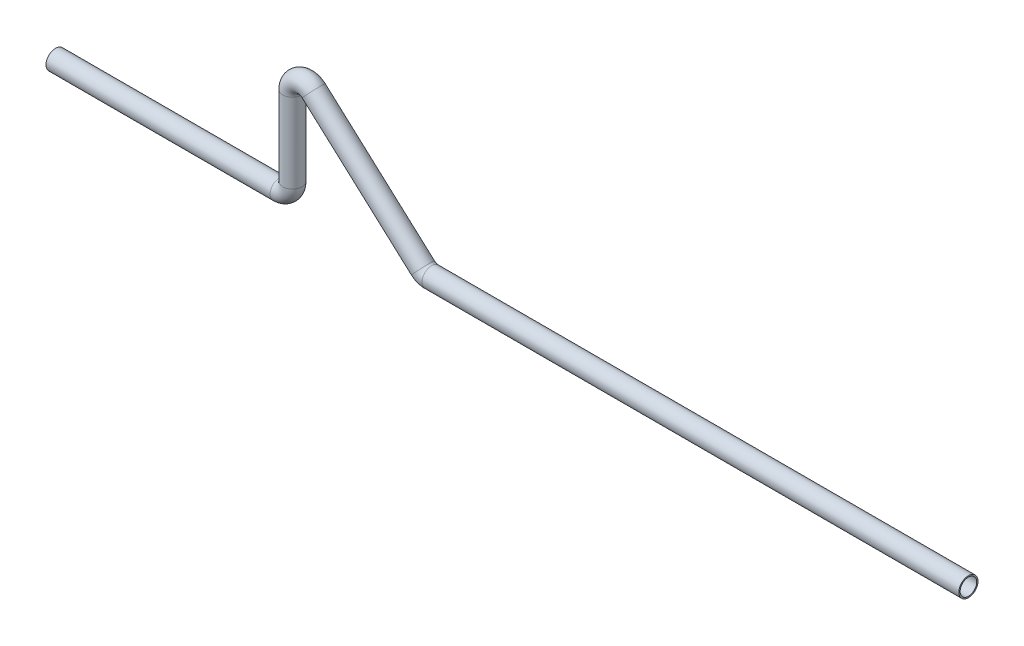
from build123d import *

# Parameters (mm, degrees)
SWEEP_THIN1_PROFILE_R   = 15
SWEEP_THIN1_PROFILE_R_2 = 13


with BuildPart() as part:
    # Sweep-Thin1: sweep along a curve in space
    with BuildLine() as sweep_thin1_path:
        Line((-2125, 3135.002861913, 100.000000001), (-1773.960788665, 3135.002861913, 100.000000001))
        ThreePointArc((-1773.960788665, 3135.002861913, 100.000000001), (-1759.818653041, 3140.860726289, 100.000000001), (-1753.960788665, 3155.002861913, 100.000000001))
        Line((-1753.960788665, 3155.002861913, 100.000000001), (-1753.960788665, 3279.60825422, 100.000000001))
        ThreePointArc((-1753.960788665, 3279.60825422, 100.000000001), (-1742.076616051, 3297.887568918, 100), (-1720.547454081, 3294.443430502, 100))
        Line((-1720.547454081, 3294.443430502, 100), (-1549.428219579, 3139.724706402, 99.999999999))
        ThreePointArc((-1536.014884995, 3134.559882685, 99.999999999), (-1543.201555794, 3135.895698727, 99.999999999), (-1549.428219579, 3139.724706402, 99.999999999))
        Line((-1536.014884995, 3134.559882685, 99.999999999), (-694.909600267, 3134.559882685, 99.999999999))
    # Sweep-Thin1 profile (on start of the path) → Sweep-Thin1 (sweep)
    with BuildSketch(Plane(origin=(-2125, 3135.002861913, 100.000000001), x_dir=(0, 0, 1), z_dir=(1, 0, 0))):
        Circle(SWEEP_THIN1_PROFILE_R)
        Circle(SWEEP_THIN1_PROFILE_R_2, mode=Mode.SUBTRACT)
    sweep(path=sweep_thin1_path.line)


solid = part.part
